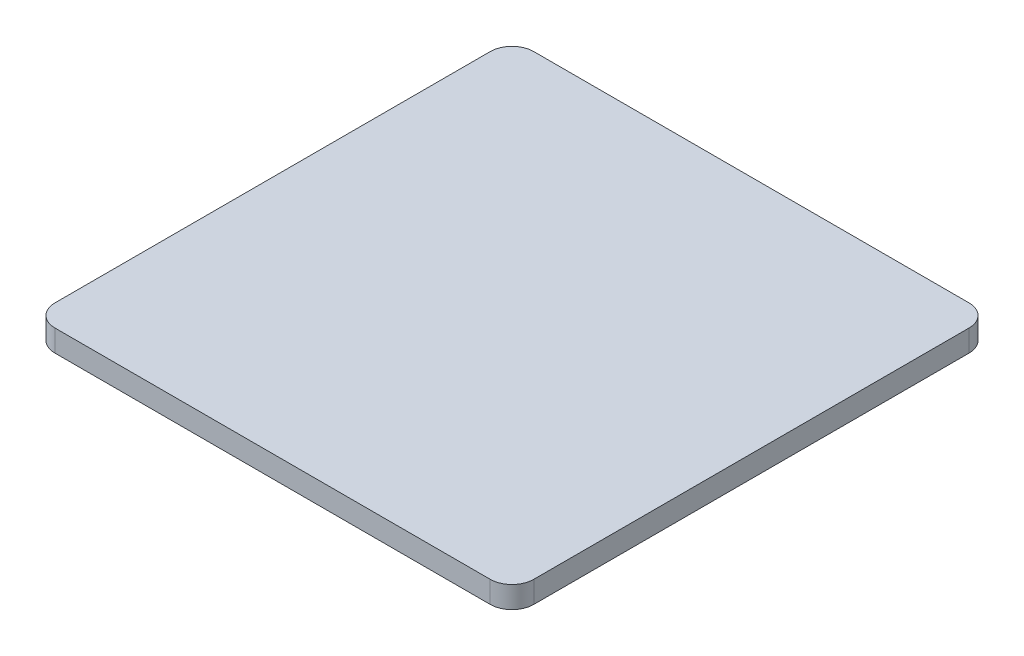
SolidWorks part; units mm, degrees
ref_plane "前视基准面" through (0, 0, 0) normal (0, 0, 1) x (1, 0, 0)
ref_plane "上视基准面" through (0, 0, 0) normal (0, 1, 0) x (1, 0, 0)
ref_plane "右视基准面" through (0, 0, 0) normal (1, 0, 0) x (0, 0, -1)
sketch "草图1" plane through (0, 0, 0) normal (0, 1, 0) x (1, 0, 0)
  line L1 (110, -110) -> (-110, -110)
  line L2 (110, -110) -> (110, 110)
  line L3 (110, 110) -> (-110, 110)
  line L4 (-110, -110) -> (-110, 110)
  line L5 (110, -110) -> (-110, 110) construction
  line L6 (110, 110) -> (-110, -110) construction
  point P0 (0, 0)
  dimension "D1" = 220
  dimension "D2" = 220
extrude "凸台-拉伸1" add sketch "草图1" along normal mid plane 10
fillet "圆角1" radius 10 4 edges at (-110, 0, -110) (-110, 0, 110) (110, 0, 110) (110, 0, -110)
sketch "草图2" plane through (0, -5, 0) normal (0, -1, 0) x (1, 0, 0)
  circle A0 centre (0, 0) radius 20.1699
